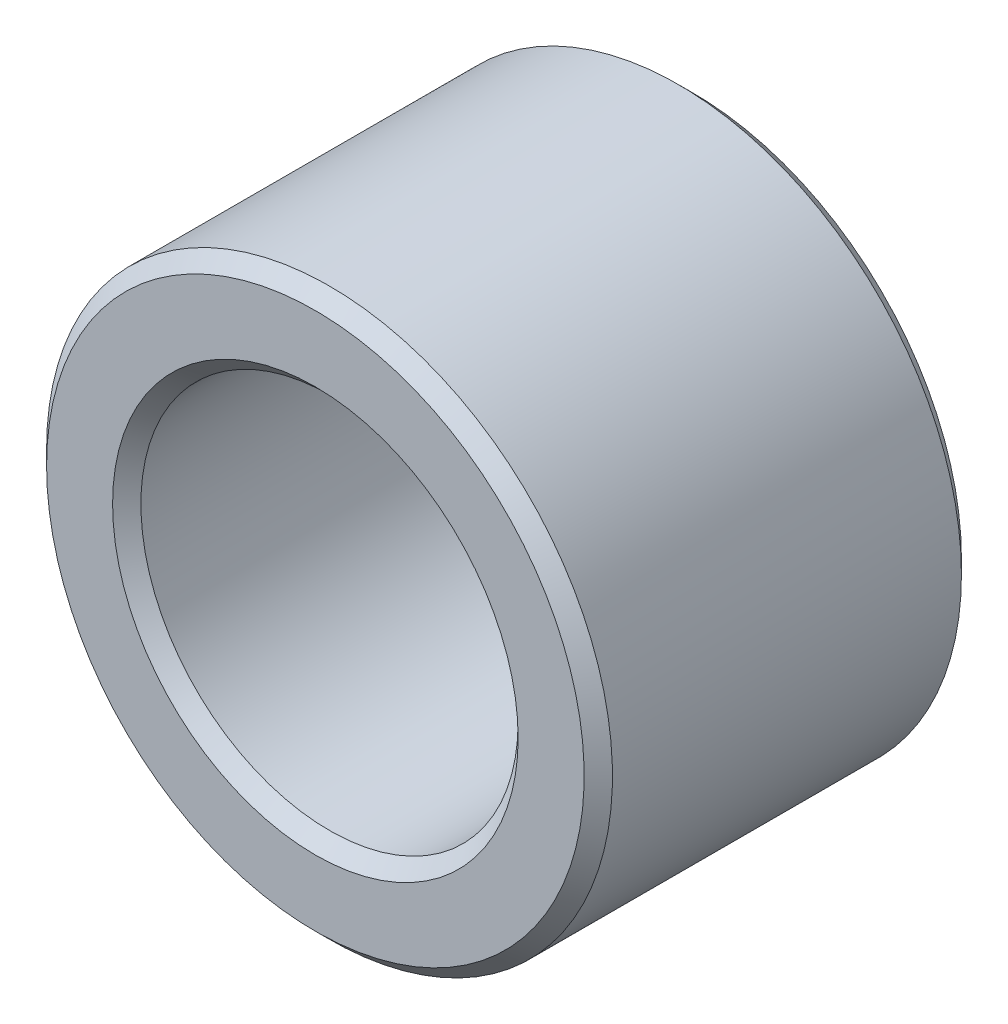
SolidWorks part; units mm, degrees
material "黄铜"
ref_plane "前视基准面" through (0, 0, 0) normal (0, 0, 1) x (1, 0, 0)
ref_plane "上视基准面" through (0, 0, 0) normal (0, 1, 0) x (1, 0, 0)
ref_plane "右视基准面" through (0, 0, 0) normal (1, 0, 0) x (0, 0, -1)
sketch "草图1" plane through (0, 0, 0) normal (0, 0, 1) x (1, 0, 0)
  circle A0 centre (0, 0) radius 4
  circle A1 centre (0, 0) radius 6
  dimension "D1" = 12
  dimension "D2" = 8
extrude "凸台-拉伸1" add sketch "草图1" along normal mid plane 8
chamfer "倒角1" distance 0.3 angle 45 4 edges at (4, 0, -4) (6, 0, -4) (4, 0, 4) (6, 0, 4)
